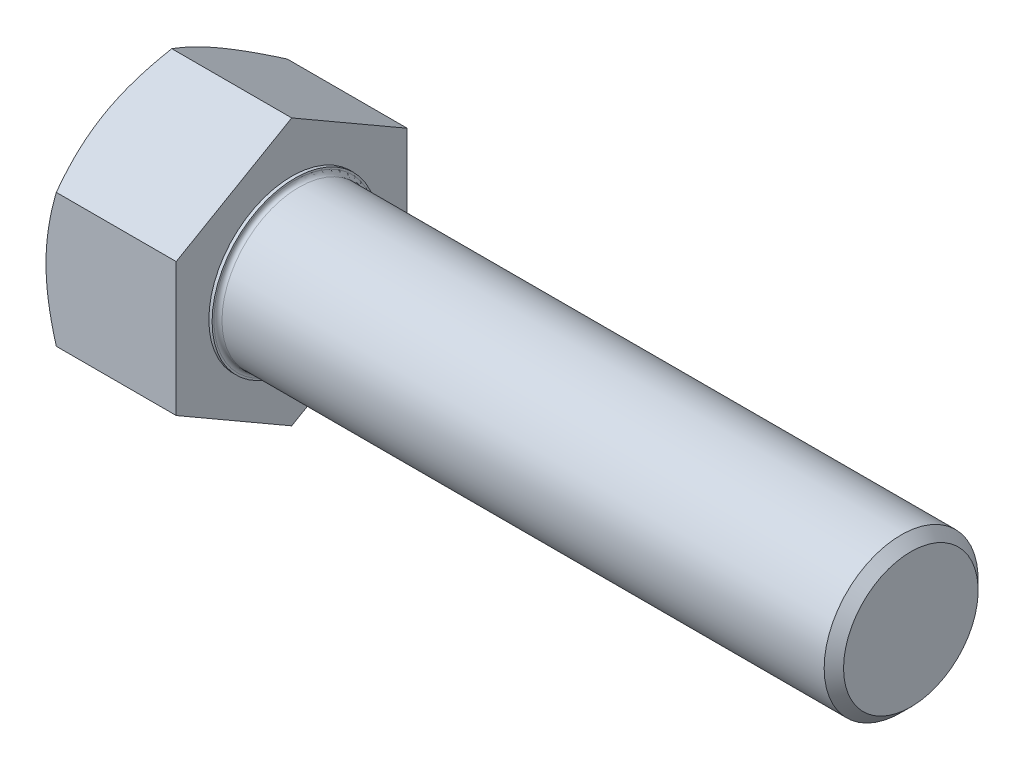
SolidWorks part; units mm, degrees
material "SAE2"
ref_plane "Front plane" through (0, 0, 0) normal (0, 0, 1) x (1, 0, 0)
ref_plane "Top plane" through (0, 0, 0) normal (0, 1, 0) x (1, 0, 0)
ref_plane "Right plane" through (0, 0, 0) normal (1, 0, 0) x (0, 0, -1)
sketch "Sketch1" plane through (0, 0, 0) normal (1, 0, 0) x (0, 0, -1)
  line L0 (28.575, 16.4978) -> (28.575, -16.4978)
  line L1 (-28.575, 16.4978) -> (-28.575, -16.4978)
  line L2 (28.575, -16.4978) -> (0, -32.9956)
  line L3 (0, -32.9956) -> (-28.575, -16.4978)
  line L4 (28.575, 16.4978) -> (0, 32.9956)
  line L5 (0, 32.9956) -> (-28.575, 16.4978)
  line L7 (-10.2574, 0) -> (16.1684, 0) construction
  dimension "D1" = 120
  dimension "s" = 57.15
  dimension "D2" = 120
  dimension "D3" = 120
extrude "Base-Extrude" add sketch "Sketch1" along normal blind 33.02
sketch "Sketch2" plane through (0, 0, 0) normal (0, 0, 1) x (1, 0, 0)
  line L0 (0, 16.4978) -> (0, -16.4978) construction
  line L1 (0, 0) -> (185.42, 0)
  line L2 (0, 0) -> (0, 19.05)
  line L3 (0, 19.05) -> (27.8072, 19.05)
  line L4 (185.42, 0) -> (185.42, 13.8)
  line L5 (33.02, 32.9956) -> (33.02, 16.4978) construction
  line L7 (0, 0) -> (96.52, 0) construction
  line L8 (185.42, -13.8) -> (27.8072, -19.05) construction
  line L9 (0, -19.05) -> (27.8072, -19.05) construction
  line L10 (36.02, 15.24) -> (36.02, -1.27) construction
  line L11 (115.57, 15.24) -> (115.57, -1.27) construction
  line L12 (33.02, 16.4978) -> (33.02, -16.4978) construction
  line L13 (27.8072, 19.05) -> (185.42, 19.05)
  line L14 (185.42, 19.05) -> (185.42, 13.8)
  dimension "l" = 152.4
  dimension "m" = 38.1
  dimension "Minor_dia" = 27.6
  dimension "p" = 3
  dimension "h" = 69.85
revolve "Boss-Revolve1" add sketch "Sketch2" angle 360 about L7
cosmetic thread "Helix1" parameters "Thread_length"=82.55, "Thread_minor"=26.9875
sketch "Sketch3" plane through (0, 0, 0) normal (0, 0, 1) x (1, 0, 0)
  line L0 (0, 28.575) -> (5.439, 37.9956)
  line L1 (0, 32.9956) -> (0, 16.4978) construction
  line L2 (5.439, 37.9956) -> (5.439, 42.9956)
  line L3 (5.439, 42.9956) -> (-10, 42.9956)
  line L4 (-10, 42.9956) -> (-10, 28.575)
  line L5 (-10, 28.575) -> (0, 28.575)
  line L6 (0, 0) -> (99.06, 0) construction
  line L7 (33.02, 32.9956) -> (0, 32.9956) construction
  dimension "D1" = 28.575
  dimension "D2" = 5
  dimension "D3" = 10
  dimension "D4" = 5
  dimension "Head_ch_ang" = 30
revolve "Cut-Revolve1" cut sketch "Sketch3" angle 360 about L6
sketch "Sketch5" plane through (0, 0, 0) normal (0, 0, 1) x (1, 0, 0)
  line L0 (33.02, 30.66) -> (28.7848, 37.9956)
  line L1 (33.02, 32.9956) -> (33.02, 16.4978) construction
  line L2 (28.7848, 37.9956) -> (28.7848, 42.9956)
  line L3 (28.7848, 42.9956) -> (38.7848, 42.9956)
  line L4 (38.7848, 42.9956) -> (38.7848, 30.66)
  line L5 (38.7848, 30.66) -> (33.02, 30.66)
  line L7 (33.02, 32.9956) -> (2.5522, 32.9956) construction
  line L8 (0, 0) -> (99.06, 0) construction
  line L9 (0, 0) -> (99.06, 0) construction
  dimension "D1" = 30.66
  dimension "D2" = 5
  dimension "D3" = 10
  dimension "Head_ch_ang" = 30
  dimension "D4" = 5
revolve "Cut-Revolve2" [suppressed] cut sketch "Sketch5" angle 360 about L8
sketch "Sketch4" plane through (0, 0, 0) normal (0, 0, 1) x (1, 0, 0)
  line L1 (33.02, 32.9956) -> (33.02, 16.4978) construction
  line L2 (33.02, 20.5) -> (32.22, 20.5)
  line L3 (33.02, 20.5) -> (33.02, 42.9956)
  line L4 (33.02, 42.9956) -> (32.22, 42.9956)
  line L5 (0, 0) -> (95.25, 0) construction
  line L6 (0, 0) -> (96.52, 0) construction
  line L7 (32.22, 20.5) -> (32.22, 42.9956)
  line L8 (33.02, 32.9956) -> (2.5522, 32.9956) construction
  dimension "D1" = 41
  dimension "D2" = 10
  dimension "c" = 0.8
revolve "Cut-Revolve3" cut sketch "Sketch4" angle 360 about L5
chamfer "Chamfer" distance 2.4 angle 45 1 edges at (185.42, 0, 19.05)
fillet "Fillet" radius 1 1 edges at (33.02, 0, -19.05)
sketch "Sketch6" plane through (0, 0, 0) normal (0, 0, 1) x (1, 0, 0)
  line L0 (57, -10.902) -> (55.5, -13.5)
  line L1 (57, -10.902) -> (58.5, -13.5)
  line L2 (58.5, -13.5) -> (58.5, -16.875)
  line L3 (-3.175, 0) -> (5.1513, 0) construction
  line L5 (58.5, -16.875) -> (55.5, -16.875)
  line L6 (55.5, -16.875) -> (55.5, -13.5)
  dimension "Thread_minor" = 21.804
  dimension "Diameter" = 27
  dimension "Start" = 57
  dimension "SideAngle" = 60
  dimension "VeeAngle" = 60
  dimension "Overcut" = 33.75
revolve "Cut-Revolve4" [suppressed] cut sketch "Sketch6" angle 360 about L3
pattern_linear "LPattern1" [suppressed]
